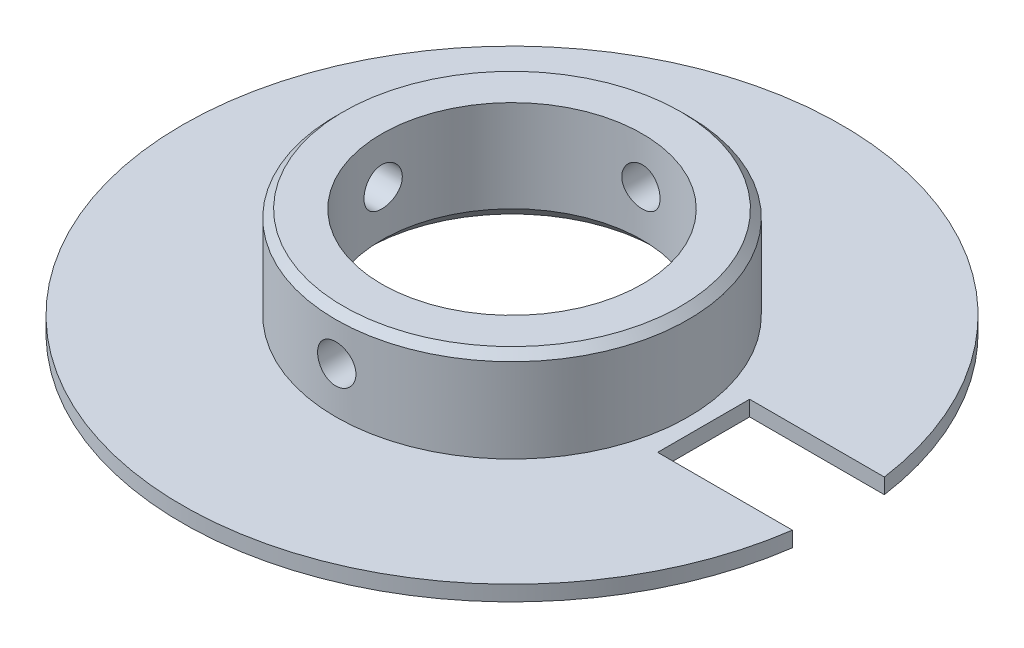
SolidWorks part; units mm, degrees
material "A6061"
ref_plane "Front Plane" through (0, 0, 0) normal (0, 0, 1) x (1, 0, 0)
ref_plane "Top Plane" through (0, 0, 0) normal (0, 1, 0) x (1, 0, 0)
ref_plane "Right Plane" through (0, 0, 0) normal (1, 0, 0) x (0, 0, -1)
sketch "Sketch2" plane through (0, 0, 0) normal (1, 0, 0) x (0, 0, -1)
  line L0 (0, 67.2949) -> (0, -48.052) construction
  line L1 (8.5, 0) -> (21.5, 0)
  line L2 (21.5, 0) -> (21.5, 1)
  line L3 (21.5, 1) -> (11.5, 1)
  line L4 (11.5, 1) -> (11.5, 7)
  line L5 (11.5, 7) -> (8.5, 7)
  line L6 (8.5, 0) -> (8.5, 7)
  dimension "D1" = 8.5
  dimension "D2" = 13
  dimension "D3" = 3
  dimension "D4" = 7
  dimension "D5" = 1
revolve "Revolve1" add sketch "Sketch2" angle 360 about L0
chamfer "Chamfer1" distance 1 angle 45 1 edges at (0, 0, 8.5)
sketch "Sketch7" plane through (0, 1, 0) normal (0, 1, 0) x (1, 0, 0)
  line L1 (12.5, 3) -> (23.7568, 3)
  line L2 (0, 0) -> (35.9898, 0) construction
  line L3 (12.5, 3) -> (12.5, -3)
  line L4 (12.5, -3) -> (23.7568, -3)
  line L5 (23.7568, 3) -> (23.7568, -3)
  dimension "D1" = 6
  dimension "D2" = 12.5
extrude "Cut-Extrude1" cut sketch "Sketch7" against normal blind 10
hole_wizard "M3 Tapped Hole2" positions "Sketch10" profile "Sketch9" tap size "M3" standard "Gb"
sketch "Sketch10" plane through (0, 0, 0) normal (1, 0, 0) x (0, 0, -1)
  line L0 (0, 0) -> (0, 11.8505) construction
  line L3 (8.5, 7) -> (-8.5, 7) construction
  point P0 (0, 4)
  dimension "D1" = 3
sketch "Sketch9" plane through (0, 4, 0) normal (0, 1, 0) x (0, 0, -1)
  line L0 (0, 0) -> (0, 21.5)
  line L1 (0, 21.5) -> (1.25, 21.5)
  line L2 (1.25, 21.5) -> (1.25, 0)
  line L5 (1.25, 0) -> (0, 0)
  line L11 (0, -6.35) -> (0, 107.95) construction
  dimension "通孔螺纹孔钻头直径" = 2.5
  dimension "通孔螺纹孔钻头深度" = 21.5
cosmetic thread "Cosmetic Thread2" parameters "D2"=3
chamfer "Chamfer2" distance 0.5 angle 45 1 edges at (0, 7, 11.5)
pattern_circular "CirPattern1" count 4 over 360 about axis through (0, 67.2949, 0) along (0, 1, 0) skipping 2 of "M3 Tapped Hole2"
